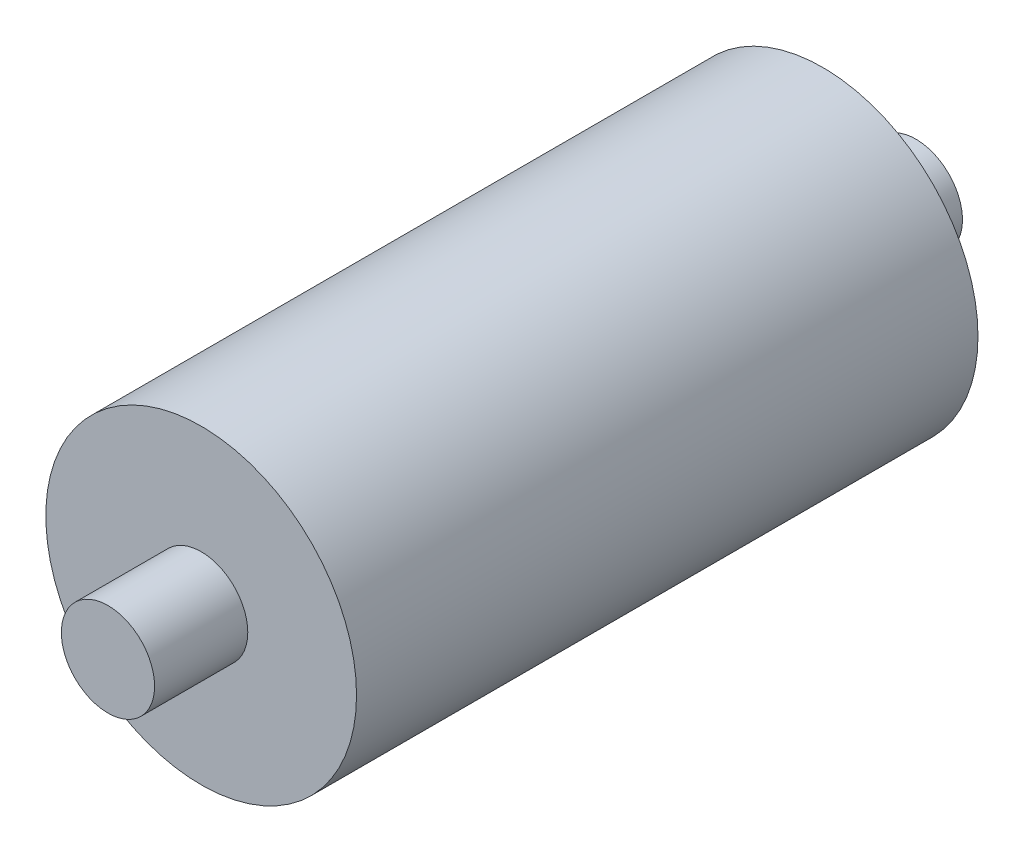
SolidWorks part; units mm, degrees
ref_plane "前视基准面" through (0, 0, 0) normal (0, 0, 1) x (1, 0, 0)
ref_plane "上视基准面" through (0, 0, 0) normal (0, 1, 0) x (1, 0, 0)
ref_plane "右视基准面" through (0, 0, 0) normal (1, 0, 0) x (0, 0, -1)
sketch "草图1" plane through (0, 0, 0) normal (0, 0, 1) x (1, 0, 0)
  circle A0 centre (0, 0) radius 25
  dimension "D1" = 50
extrude "凸台-拉伸1" add sketch "草图1" along normal blind 100
sketch "草图2" plane through (0, 0, 100) normal (0, 0, 1) x (1, 0, 0)
  circle A0 centre (0, 0) radius 7.5
  dimension "D1" = 15
extrude "凸台-拉伸2" add sketch "草图2" along normal blind 15
sketch "草图3" plane through (0, 0, 0) normal (0, 0, -1) x (-1, 0, 0)
  circle A0 centre (0, 0) radius 7.5
  dimension "D1" = 15
extrude "凸台-拉伸3" add sketch "草图3" along normal blind 15
